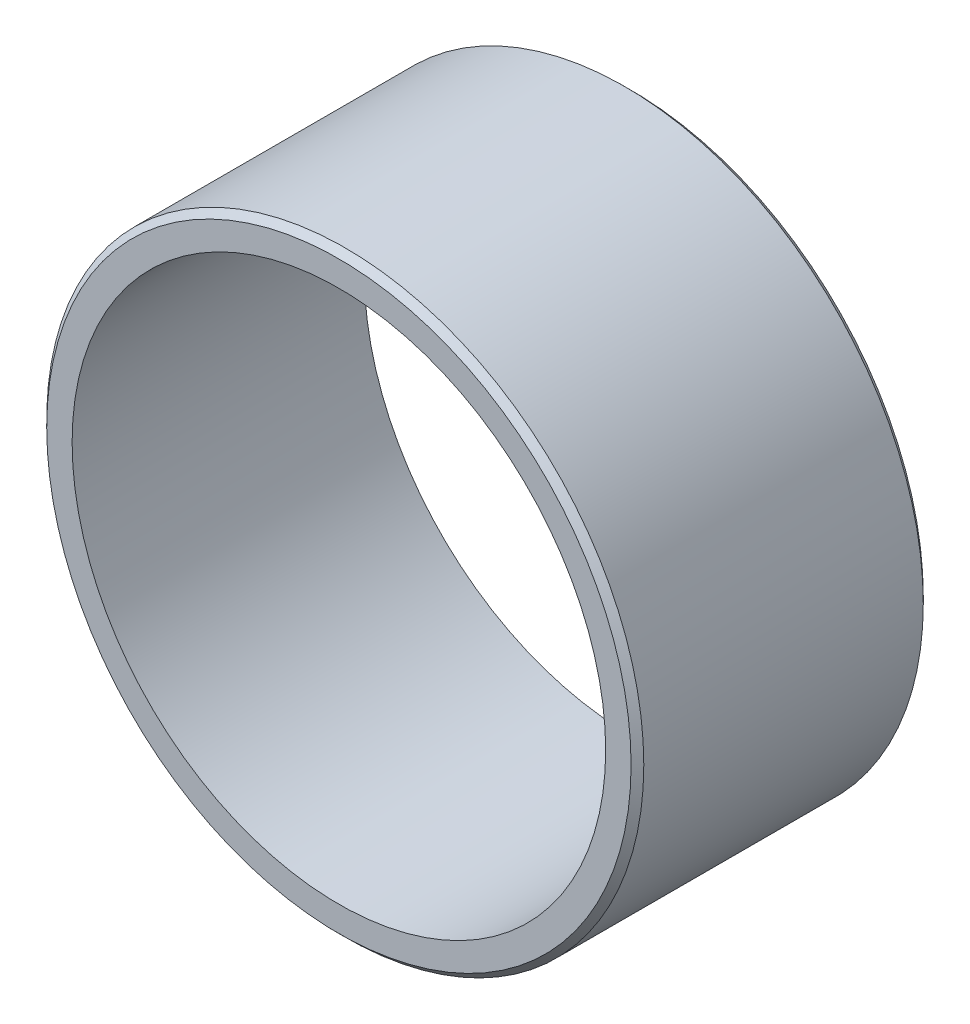
SolidWorks part; units mm, degrees
ref_plane "Front Plane" through (0, 0, 0) normal (0, 0, 1) x (1, 0, 0)
ref_plane "Top Plane" through (0, 0, 0) normal (0, 1, 0) x (1, 0, 0)
ref_plane "Right Plane" through (0, 0, 0) normal (1, 0, 0) x (0, 0, -1)
sketch "Sketch1" plane through (0, 0, 0) normal (0, 0, 1) x (1, 0, 0)
  circle A0 centre (0, 0) radius 23.5
  circle A1 centre (0, 0) radius 21
  dimension "D1" = 47
  dimension "D2" = 42
extrude "Boss-Extrude1" add sketch "Sketch1" along normal blind 23
chamfer "Chamfer1" distance 0.5 angle 45 2 edges at (23.5, 0, 23) (23.5, 0, 0)
